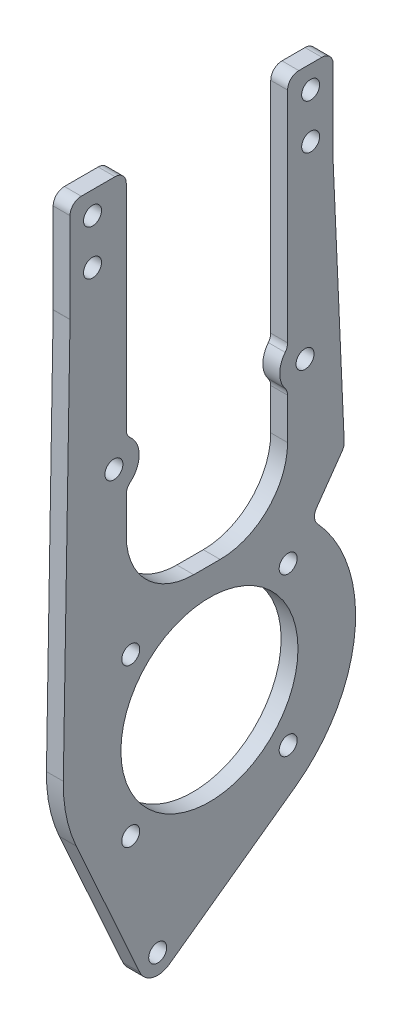
from build123d import *

# Parameters (mm, degrees)
SKETCH_1_R          = 15.75
SKETCH_1_R_2        = 1.6
EXTRUDE_1_DEPTH     = 3
SKETCH_2_W          = 28.7
SKETCH_2_H          = 68.308962896
CUT_EXTRUDE_1_DEPTH = 93.750249245
FILLET_1_R          = 12
SKETCH_4_R          = 1.6
CUT_EXTRUDE_2_DEPTH = 93.750249245
SKETCH_5_R          = 4.5
SKETCH_5_R_2        = 1.6
EXTRUDE_2_DEPTH     = 3
FILLET_2_R          = 2


with BuildPart() as part:
    # 草图1 → 凸台-拉伸1 (new body)
    with BuildSketch(Plane(origin=(0, 0, 0), x_dir=(0, 0, -1), z_dir=(1, 0, 0))):
        with BuildLine():
            Line((18.093011091, 18.671983014), (24, 27.077468597))
            Line((24, 27.077468597), (22, 71.98094591))
            Line((22, 71.98094591), (22, 88.98094591))
            Line((22, 88.98094591), (-24.8, 88.98094591))
            Line((-24.8, 88.98094591), (-24.8, 70.98094591))
            Line((-24.8, 70.98094591), (-25.996262077, 0.440860573))
            ThreePointArc((-25.996262077, 0.440860573), (9.935230264, -24.026884933), (18.093011091, 18.671983014))
        make_face()
        Circle(SKETCH_1_R, mode=Mode.SUBTRACT)
        with Locations((14.000714267, 14.000714267)):
            Circle(SKETCH_1_R_2, mode=Mode.SUBTRACT)
        with Locations((14.000714267, -14.000714267)):
            Circle(SKETCH_1_R_2, mode=Mode.SUBTRACT)
        with Locations((-14.000714267, -14.000714267)):
            Circle(SKETCH_1_R_2, mode=Mode.SUBTRACT)
        with Locations((-14.000714267, 14.000714267)):
            Circle(SKETCH_1_R_2, mode=Mode.SUBTRACT)
        with Locations((-20.8, 84.98094591)):
            Circle(SKETCH_1_R_2, mode=Mode.SUBTRACT)
        with Locations((-20.8, 76.98094591)):
            Circle(SKETCH_1_R_2, mode=Mode.SUBTRACT)
        with Locations((18, 84.98094591)):
            Circle(SKETCH_1_R_2, mode=Mode.SUBTRACT)
        with Locations((18, 76.98094591)):
            Circle(SKETCH_1_R_2, mode=Mode.SUBTRACT)
    extrude(amount=EXTRUDE_1_DEPTH)

    # 草图2 → 切除-拉伸1 (cut, through all)
    with BuildSketch(Plane.ZY):
        with Locations((0.45, 54.826464462)):
            Rectangle(SKETCH_2_W, SKETCH_2_H)
    extrude(amount=-CUT_EXTRUDE_1_DEPTH, mode=Mode.SUBTRACT)

    # 圆角1
    fillet_1_edges = [part.edges().sort_by_distance(p)[0] for p in [
        (1.5, 20.671983014, -13.9),
        (1.5, 20.671983014, 14.8),
    ]]
    fillet(fillet_1_edges, radius=FILLET_1_R)

    # 草图4 → 切除-拉伸2 (cut, through all)
    with BuildSketch(Plane(origin=(3, 0, 0), x_dir=(0, 0, -1), z_dir=(1, 0, 0))):
        with Locations((-17, 44.000714267)):
            Circle(SKETCH_4_R)
        with Locations((17, 44.000714267)):
            Circle(SKETCH_4_R)
    extrude(amount=-CUT_EXTRUDE_2_DEPTH, mode=Mode.SUBTRACT)

    # 草图5 → 凸台-拉伸2 (add)
    # profile 1 of 3: a face of its own
    with BuildSketch(Plane(origin=(3, 0, 0), x_dir=(0, 0, -1), z_dir=(1, 0, 0))):
        with Locations((-17, 44.000714267)):
            Circle(SKETCH_5_R)
        with Locations((-17, 44.000714267)):
            Circle(SKETCH_5_R_2, mode=Mode.SUBTRACT)
    # profile 2 of 3: a face of its own
    with BuildSketch(Plane(origin=(3, 0, 0), x_dir=(0, 0, -1), z_dir=(1, 0, 0))):
        with Locations((17, 44.000714267)):
            Circle(SKETCH_5_R)
        with Locations((17, 44.000714267)):
            Circle(SKETCH_5_R_2, mode=Mode.SUBTRACT)
    # profile 3 of 3: a face of its own
    with BuildSketch(Plane(origin=(3, 0, 0), x_dir=(0, 0, -1), z_dir=(1, 0, 0))):
        with BuildLine():
            Line((-12.394227472, -35.784446941), (-23.70501151, -10.680469528))
            ThreePointArc((-23.70501151, -10.680469528), (-6.729295173, -25.114071484), (15.1889074, -21.10206369))
            Line((15.1889074, -21.10206369), (-7.158507619, -37.187353847))
            ThreePointArc((-7.158507619, -37.187353847), (-10.109034889, -37.72743182), (-12.394227472, -35.784446941))
        make_face()
        with Locations((-9.203168231, -34.346691428)):
            Circle(SKETCH_5_R_2, mode=Mode.SUBTRACT)
    extrude(amount=-EXTRUDE_2_DEPTH)

    # 圆角2
    fillet_2_edges = [part.edges().sort_by_distance(p)[0] for p in [
        (1.5, 47.926271553, 14.8),
        (1.5, 40.075156982, 14.8),
        (1.5, 70.98094591, 24.8),
        (1.5, 88.98094591, 24.8),
        (1.5, 88.98094591, -22),
        (1.5, 71.98094591, -22),
        (1.5, 27.077468597, -24),
        (1.5, 40.738812981, -13.9),
        (1.5, 18.671983014, -18.093011091),
        (1.5, 47.262615554, -13.9),
        (1.5, 88.98094591, -13.9),
        (1.5, 88.98094591, 14.8),
    ]]
    fillet(fillet_2_edges, radius=FILLET_2_R)


solid = part.part
